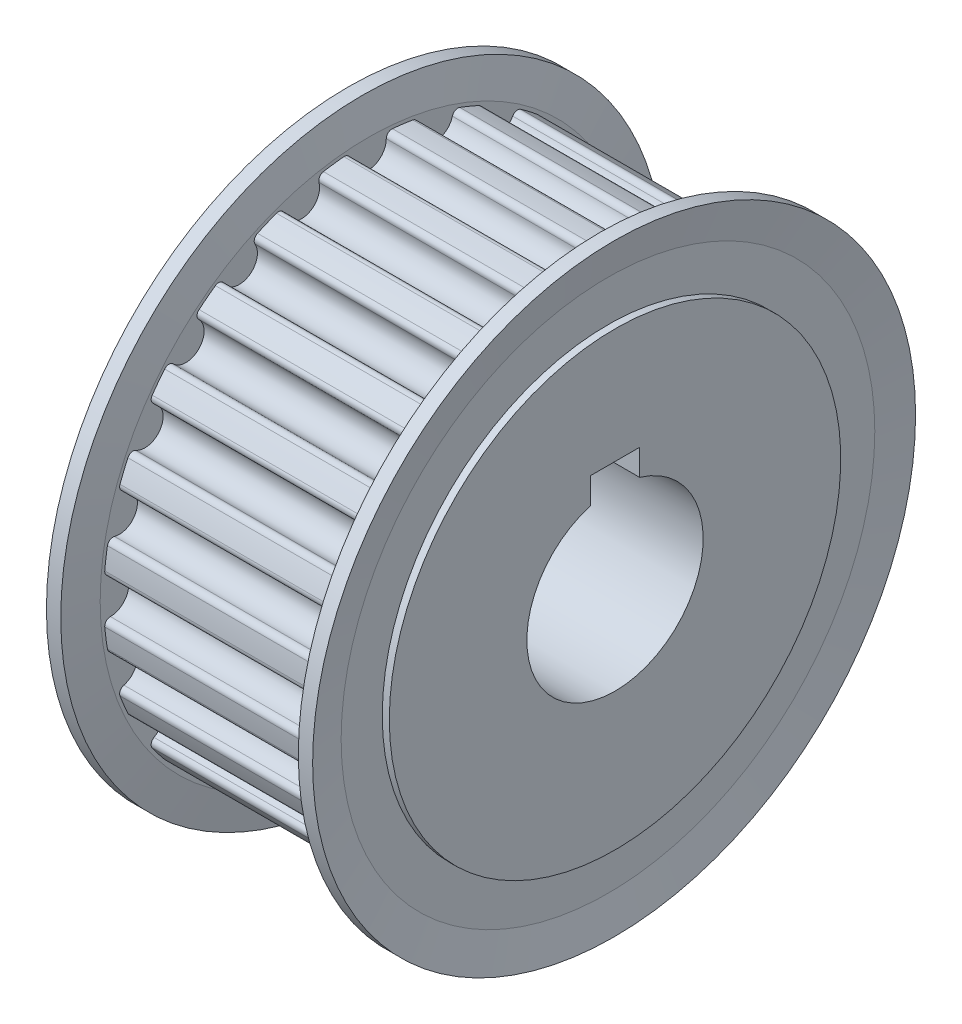
from build123d import *

# Parameters (mm, degrees)
SKETCH_2_W               = 7
SKETCH_2_H               = 15.7
CUT_EXTRUDE_1_DEPTH      = 72.396184772
CUT_EXTRUDE_START        = -32
CUT_EXTRUDE_2_DEPTH      = 32
PATTERN_CIRCULAR_1_COUNT = 24


with BuildPart() as part:
    # 草图1 → 旋转1 (revolve)
    with BuildSketch(Plane.XY, mode=Mode.PRIVATE) as revolve_1_sk:
        Polygon((19, 32), (18.87, 32), (18, 32), (16, 32), (16, 37.5), (-16, 37.5), (-16, 32), (-18, 32), (-18.87, 32), (-19, 32), (-19, 12.5), (19, 12.5), align=None)
        Polygon((-16, 32), (-16, 37.5), (-16, 37.99), (-16.84, 42.74), (-18.87, 42.74), (-18, 37.83), (-18, 32), align=None)
        Polygon((18, 37.83), (18.87, 42.74), (16.84, 42.74), (16, 37.99), (16, 37.5), (16, 32), (18, 32), align=None)
    revolve(revolve_1_sk.sketch.rotate(Axis((-24.150544069, 0, 0), (1, 0, 0)), 90), axis=Axis((-24.150544069, 0, 0), (1, 0, 0)))

    # 草图2 → 切除-拉伸1 (cut, through all)
    with BuildSketch(Plane(origin=(19, 0, 0), x_dir=(0, 0, -1), z_dir=(1, 0, 0))):
        with Locations((0, 7.85)):
            Rectangle(SKETCH_2_W, SKETCH_2_H)
    extrude(amount=-CUT_EXTRUDE_1_DEPTH, mode=Mode.SUBTRACT)

    # 草图4 → 切除-拉伸2 (cut)
    with BuildSketch(Plane(origin=(16, 0, 0), x_dir=(0, 0, -1), z_dir=(1, 0, 0)).offset(CUT_EXTRUDE_START)):
        with BuildLine():
            ThreePointArc((3.44342661, 37.341569506), (0, 37.5), (-3.44342661, 37.341569506))
            ThreePointArc((-3.44342661, 37.341569506), (-2.829568925, 37.134839255), (-2.569974713, 36.541400548))
            ThreePointArc((-2.569974713, 36.541400548), (0, 33.96), (2.569974713, 36.541400548))
            ThreePointArc((2.569974713, 36.541400548), (2.829568925, 37.134839255), (3.44342661, 37.341569506))
        make_face()
    cut_extrude_2 = extrude(amount=CUT_EXTRUDE_2_DEPTH, mode=Mode.SUBTRACT)

    # 阵列(圆周)1: 切除-拉伸2 ×24 about axis
    pattern_circular_1_axis = Axis((0, 0, 0), (1, 0, 0))
    for i in range(1, PATTERN_CIRCULAR_1_COUNT):
        add(cut_extrude_2.rotate(pattern_circular_1_axis, i * 360 / PATTERN_CIRCULAR_1_COUNT), mode=Mode.SUBTRACT)


solid = part.part
